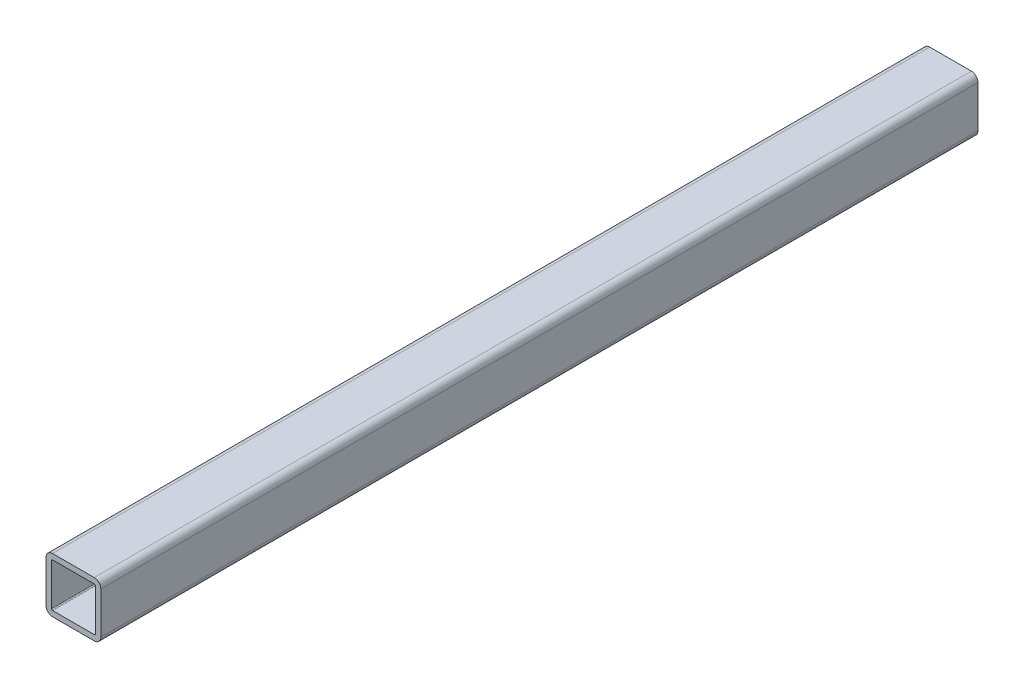
from build123d import *

# Parameters (mm, degrees)
BOSS_EXTRUDE1_DEPTH = 800


with BuildPart() as part:
    # Sketch1 → Boss-Extrude1 (new body)
    with BuildSketch(Plane.XY):
        with BuildLine():
            Line((6, 0), (44, 0))
            ThreePointArc((44, 0), (48.242640687, 1.757359313), (50, 6))
            Line((50, 6), (50, 44))
            ThreePointArc((50, 44), (48.242640687, 48.242640687), (44, 50))
            Line((44, 50), (6, 50))
            ThreePointArc((6, 50), (1.757359313, 48.242640687), (0, 44))
            Line((0, 44), (0, 6))
            ThreePointArc((0, 6), (1.757359313, 1.757359313), (6, 0))
        make_face()
        with BuildLine():
            Line((6, 45), (44, 45))
            ThreePointArc((44, 45), (44.707106781, 44.707106781), (45, 44))
            Line((45, 44), (45, 6))
            ThreePointArc((45, 6), (44.707106781, 5.292893219), (44, 5))
            Line((44, 5), (6, 5))
            ThreePointArc((6, 5), (5.292893219, 5.292893219), (5, 6))
            Line((5, 6), (5, 44))
            ThreePointArc((5, 44), (5.292893219, 44.707106781), (6, 45))
        make_face(mode=Mode.SUBTRACT)
    extrude(amount=BOSS_EXTRUDE1_DEPTH)


solid = part.part
